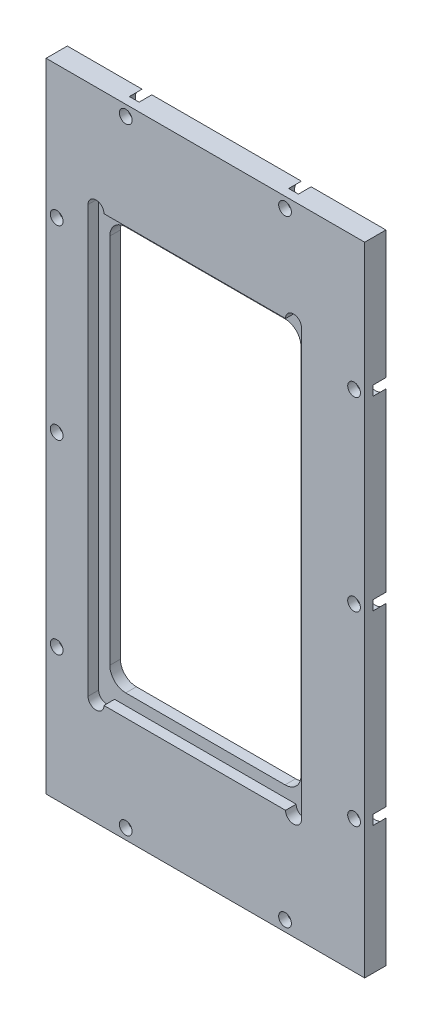
SolidWorks part; units mm, degrees
material "6061Al"
ref_plane "前视基准面" through (0, 0, 0) normal (0, 0, 1) x (1, 0, 0)
ref_plane "上视基准面" through (0, 0, 0) normal (0, 1, 0) x (1, 0, 0)
ref_plane "右视基准面" through (0, 0, 0) normal (1, 0, 0) x (0, 0, -1)
sketch "草图1" plane through (0, 0, 0) normal (0, 0, 1) x (1, 0, 0)
  line L1 (-30, -60) -> (30, -60)
  line L2 (-30, -60) -> (-30, 60)
  line L3 (-30, 60) -> (30, 60)
  line L4 (30, -60) -> (30, 60)
  line L5 (-30, -60) -> (30, 60) construction
  line L6 (-30, 60) -> (30, -60) construction
  point P0 (0, 0)
  dimension "D1" = 120
  dimension "D2" = 60
extrude "凸台-拉伸1" add sketch "草图1" along normal mid plane 4
sketch "草图2" plane through (0, 0, 2) normal (0, 0, 1) x (1, 0, 0)
  line L0 (0, 0) -> (30, 0) construction
  line L1 (30, -60) -> (30, 60) construction
  line L2 (-30, 60) -> (-30, -60) construction
  line L3 (-20, 38) -> (16, 38)
  line L4 (-20, 38) -> (-20, -38)
  line L5 (-20, -38) -> (16, -38)
  line L6 (16, 38) -> (16, -38)
  dimension "D1" = 36
  dimension "D2" = 76
  dimension "D3" = 10
extrude "切除-拉伸1" cut sketch "草图2" against normal through all
sketch "草图3" plane through (0, 0, 2) normal (0, 0, 1) x (1, 0, 0)
  line L8 (18.1, 40.1) -> (-22.1, 40.1)
  line L9 (18.1, -40.1) -> (18.1, 40.1)
  line L10 (-22.1, -40.1) -> (18.1, -40.1)
  line L11 (-22.1, 40.1) -> (-22.1, -40.1)
  line L12 (18.1, 40.1) -> (-22.1, 40.1)
  line L13 (18.1, -40.1) -> (18.1, 40.1)
  line L14 (-22.1, -40.1) -> (18.1, -40.1)
  line L15 (-22.1, 40.1) -> (-22.1, -40.1)
  dimension "D1" = 2.1
extrude "切除-拉伸2" cut sketch "草图3" against normal blind 2
hole_wizard "Ø3.0 (3) 直径孔1" positions "草图4" profile "草图5" hole size "Ø3.0" standard "ISO" end condition up to next
sketch "草图4" plane through (0, 0, 2) normal (0, 0, 1) x (1, 0, 0)
  line L0 (18.1, 40.1) -> (-22.1, 40.1) construction
  line L1 (-22.1, 40.1) -> (-22.1, -40.1) construction
  line L8 (-30, 0) -> (30, 0) construction
  line L9 (-30, 60) -> (-30, -60) construction
  line L10 (30, -60) -> (30, 60) construction
  line L12 (-2, 38) -> (-2, 73.6475) construction
  line L13 (-20, 38) -> (16, 38) construction
  point P0 (-20.6, 40.1)
  point P17 (16.6, 40.1)
  point P39 (16.6, -40.1)
  point P40 (-20.6, -40.1)
  dimension "D1" = 1.5
sketch "草图5" plane through (-20.6, 40.1, 2) normal (1, 0, 0) x (0, -1, 0)
  line L0 (0, 0) -> (0, 2)
  line L1 (0, 2) -> (1.5, 2)
  line L2 (1.5, 2) -> (1.5, 0)
  line L5 (1.5, 0) -> (0, 0)
  line L11 (0, -6.35) -> (0, 107.95) construction
  dimension "通孔孔直径" = 3
  dimension "通孔孔深度" = 2
fillet "圆角1" radius 3 4 edges at (16, 38, -1) (16, -38, -1) (-20, -38, -1) (-20, 38, -1)
hole_wizard "M2 六角凹头螺钉的柱形沉头孔1" positions "草图6" profile "草图7" counterbore size "M2" standard "ISO" end condition through all
sketch "草图6" plane through (0, 0, -2) normal (0, 0, 1) x (1, 0, 0)
  point P9 (-28, 0)
  point P21 (-28, 0)
  point P23 (28, 0)
  point P27 (-15, 58)
  point P30 (15, 58)
  point P33 (-28, 35)
  point P36 (28, 35)
  point P39 (-28, -35)
  point P42 (28, -35)
  point P46 (-15, -58)
  point P49 (15, -58)
sketch "草图7" plane through (-28, 0, -2) normal (1, 0, 0) x (0, 1, 0)
  line L0 (0, 0) -> (0, 4)
  line L1 (0, 4) -> (1.2, 4)
  line L3 (1.2, 4) -> (1.2, 2.4)
  line L4 (1.2, 2.4) -> (2.2, 2.4)
  line L5 (2.2, 2.4) -> (2.2, 0)
  line L7 (2.2, 0) -> (0, 0)
  line L11 (0, -6.35) -> (0, 107.95) construction
  dimension "通孔孔直径" = 2.4
  dimension "通孔孔深度" = 4
  dimension "柱形沉头孔直径" = 4.4
  dimension "柱形沉头孔深度" = 2.4
hole_wizard "M3 螺纹孔1" positions "草图9" profile "草图10" tap size "M3" standard "ISO"
sketch "草图9" plane through (0, 0, 2) normal (0, 0, 1) x (1, 0, 0)
  line L0 (0, 60) -> (0, 74.7314) construction
  line L4 (-30, 60) -> (-30, -60) construction
  line L5 (0, 0) -> (48.9555, 0) construction
  line L7 (0, -60) -> (0, -74.7314) construction
  line L8 (30, 60) -> (-30, 60) construction
  line L9 (30, 60) -> (-30, 60) construction
  point P2 (-22.5, 56)
  point P4 (22.5, 56)
  point P6 (-26, 25)
  point P8 (26, 25)
  point P27 (26, -25)
  point P28 (-26, -25)
  point P29 (22.5, -56)
  point P30 (-22.5, -56)
  dimension "D1" = 4
  dimension "D2" = 45
  dimension "D3" = 4
  dimension "D4" = 35
sketch "草图10" plane through (-22.5, 56, 2) normal (1, 0, 0) x (0, -1, 0)
  line L0 (0, 0) -> (0, 4)
  line L1 (0, 4) -> (1.25, 4)
  line L2 (1.25, 4) -> (1.25, 0)
  line L5 (1.25, 0) -> (0, 0)
  line L11 (0, -6.35) -> (0, 107.95) construction
  dimension "通孔螺纹孔钻头直径" = 2.5
  dimension "通孔螺纹孔钻头深度" = 4
cosmetic thread "孔螺蚊线1" [suppressed] parameters "D2"=3
cosmetic thread "孔螺蚊线2" [suppressed] parameters "D2"=3
cosmetic thread "孔螺蚊线3" [suppressed] parameters "D2"=3
cosmetic thread "孔螺蚊线4" [suppressed] parameters "D2"=3
cosmetic thread "孔螺蚊线5" [suppressed] parameters "D2"=3
cosmetic thread "孔螺蚊线6" [suppressed] parameters "D2"=3
cosmetic thread "孔螺蚊线7" [suppressed] parameters "D2"=3
cosmetic thread "孔螺蚊线8" [suppressed] parameters "D2"=3
sketch "草图12" plane through (0, 0, -2) normal (0, 0, -1) x (-1, 0, 0)
  line L14 (0, 60) -> (0, -60) construction
  line L15 (-14.0835, 60) -> (14.0835, 60) construction
  line L16 (14.0835, -60) -> (-14.0835, -60) construction
  line L18 (-22.5, -50) -> (22.5, -50)
  line L19 (-22.5, -50) -> (-22.5, 50)
  line L20 (-22.5, 50) -> (22.5, 50)
  line L21 (22.5, -50) -> (22.5, 50)
  line L22 (-22.5, -50) -> (22.5, 50) construction
  line L23 (-22.5, 50) -> (22.5, -50) construction
  point P0 (0, 0)
  dimension "D1" = 100
  dimension "D2" = 45
extrude "切除-拉伸3" [suppressed] cut sketch "草图12" against normal blind 2
hole_wizard "Ø3.0 (3) 直径孔2" positions "草图13" profile "草图14" hole size "Ø3.0" standard "ISO"
sketch "草图13" [suppressed] plane through (0, 0, -2) normal (0, 0, -1) x (-1, 0, 0)
  line L0 (0, 0) -> (0, 60) construction
  line L1 (-14.0835, 60) -> (14.0835, 60) construction
  line L3 (0, 0) -> (41.6513, 0) construction
  line L5 (22.5, 50) -> (-22.5, 50) construction
  line L6 (-22.5, 50) -> (-22.5, -50) construction
  line L7 (22.5, 50) -> (-22.5, 50) construction
  line L8 (22.5, -50) -> (22.5, 50) construction
  point P0 (-21, 50)
  point P19 (21, 50)
  point P26 (21, -50)
  point P27 (-21, -50)
sketch "草图14" plane through (21, 50, -2) normal (1, 0, 0) x (0, 1, 0)
  line L0 (0, 0) -> (0, 2)
  line L1 (0, 2) -> (1.5, 2)
  line L2 (1.5, 2) -> (1.5, 0)
  line L5 (1.5, 0) -> (0, 0)
  line L11 (0, -6.35) -> (0, 107.95) construction
  dimension "通孔孔直径" = 3
  dimension "通孔孔深度" = 2
equation "\"D2@草图13\"=\"D1@草图13\""
